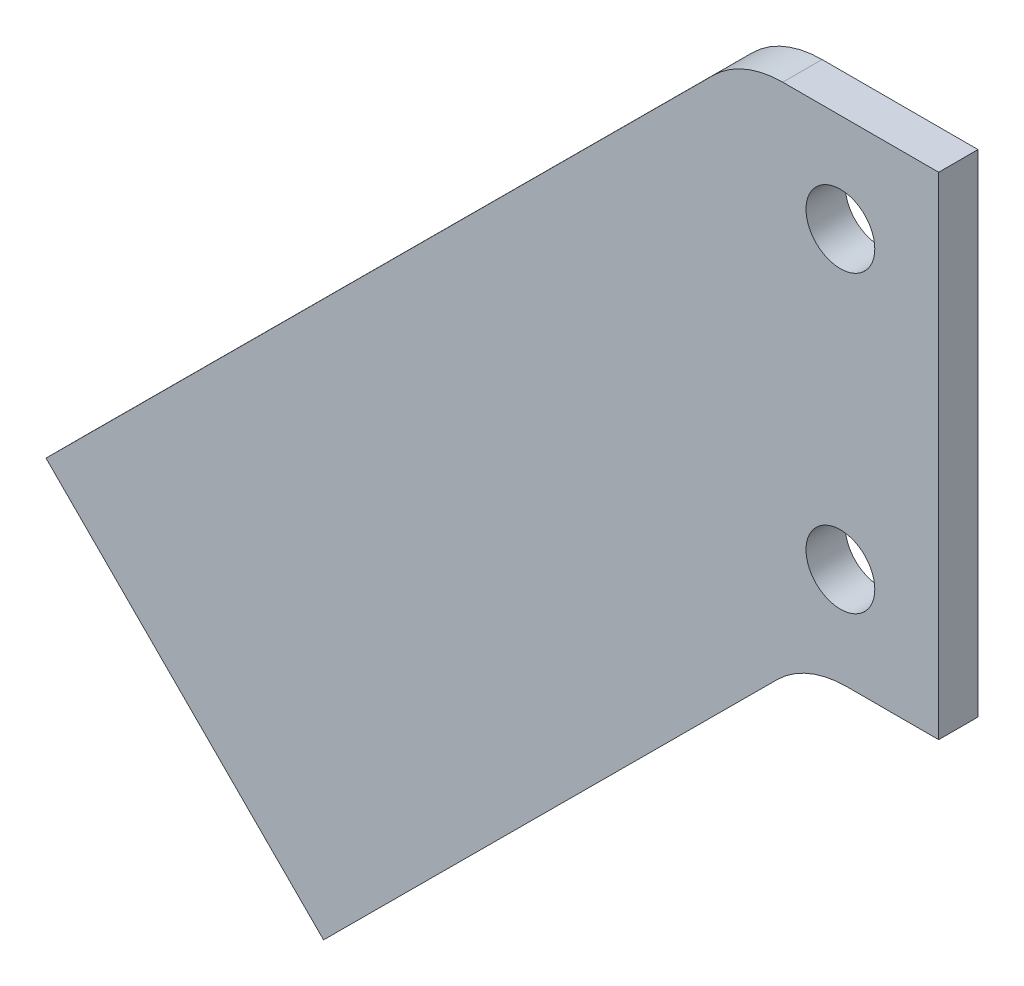
SolidWorks part; units mm, degrees
material "Q235B"
ref_plane "Front Plane" through (0, 0, 0) normal (0, 0, 1) x (1, 0, 0)
ref_plane "Top Plane" through (0, 0, 0) normal (0, 1, 0) x (1, 0, 0)
ref_plane "Right Plane" through (0, 0, 0) normal (1, 0, 0) x (0, 0, -1)
other "Configuration Table"
sketch "Sketch1" plane through (0, 0, 0) normal (0, 0, 1) x (1, 0, 0)
  line L0 (-40, 0) -> (-27, -100) construction
  line L1 (0, 0) -> (-31.7342, 0)
  line L2 (0, 0) -> (0, -100)
  line L3 (0, -100) -> (-18.7342, -100)
  line L5 (-45.854, -5.8356) -> (-181.6442, -141.1981)
  line L6 (-181.6442, -141.1981) -> (-125.165, -197.8558)
  line L7 (-125.165, -197.8558) -> (-32.854, -105.8356)
  circle A0 centre (-20, -20) radius 7
  circle A1 centre (-20, -80) radius 7
  arc A2 (-32.854, -105.8356) -> (-18.7342, -100) centre (-18.7342, -120) cw
  arc A3 (-31.7342, 0) -> (-45.854, -5.8356) centre (-31.7342, -20) ccw
  dimension "D6" = 14
  dimension "D9" = 20
  dimension "D10" = 20
  dimension "D11" = 20
  dimension "D1" = 40
  dimension "D2" = 27
  dimension "D3" = 200
  dimension "D4" = 100
  dimension "D5" = 80
  dimension "D7" = 80
  dimension "D8" = 20
extrude "Boss-Extrude1" add sketch "Sketch1" along normal blind 8
